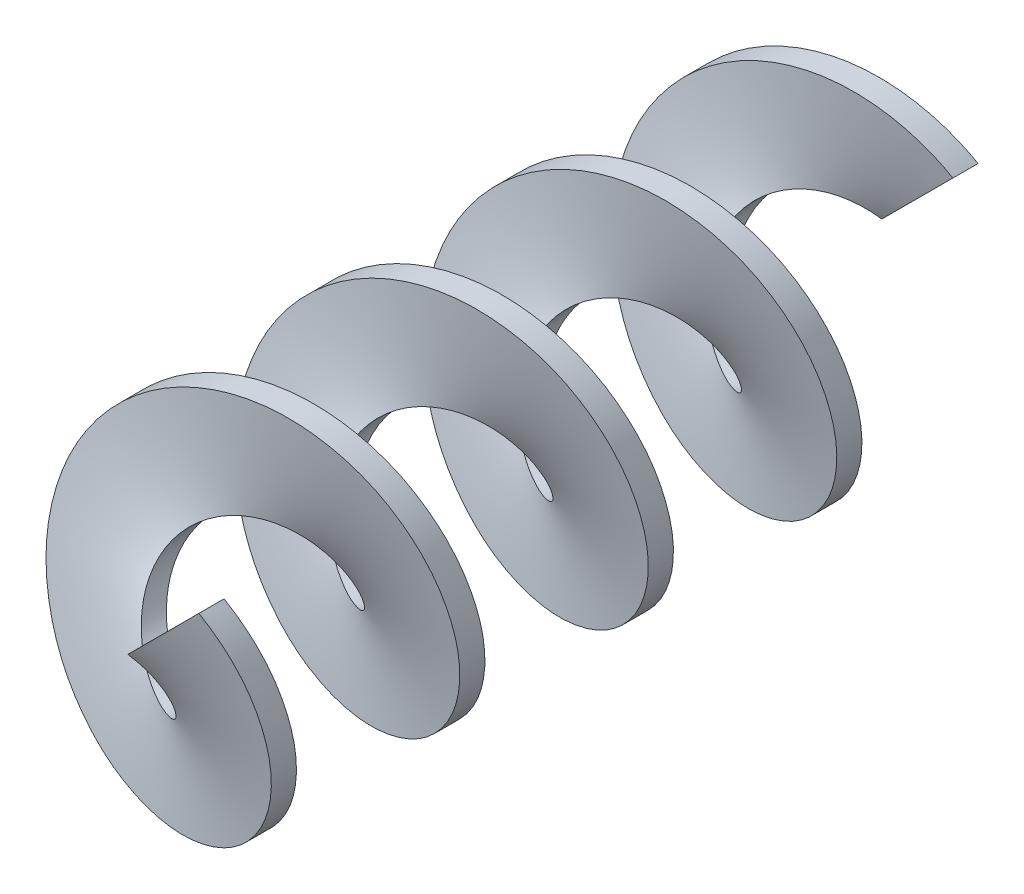
SolidWorks part; units mm, degrees
ref_plane "Front Plane" through (0, 0, 0) normal (0, 0, 1) x (1, 0, 0)
ref_plane "Top Plane" through (0, 0, 0) normal (0, 1, 0) x (1, 0, 0)
ref_plane "Right Plane" through (0, 0, 0) normal (1, 0, 0) x (0, 0, -1)
ref_plane "Plane1" through (0, 0, 15) normal (0, 0, 1) x (1, 0, 0)
sketch "Sketch2" plane through (0, 0, 15) normal (0, 0, 1) x (1, 0, 0)
  circle A0 centre (0, 0) radius 3
  dimension "D1" = 6
curve "Helix/Spiral1" pitch 3.75 height 15 turns 4
sketch "Sketch16" plane through (0, 0, 0) normal (0, 1, 0) x (1, 0, 0)
  line L1 (3.1213, -14.75) -> (1.1213, -14.75)
  line L2 (3.1213, -14.75) -> (3.1213, -15.25)
  line L3 (3.1213, -15.25) -> (1.1213, -15.25)
  line L4 (1.1213, -14.75) -> (1.1213, -15.25)
  line L5 (3.1213, -14.75) -> (1.1213, -15.25) construction
  line L6 (3.1213, -15.25) -> (1.1213, -14.75) construction
  spline S0 degree 3 poles (2.1213, -15) (2.3973, -14.9224) (2.8446, -14.7654) (3.0779, -14.5313) (2.8439, -14.2969) (2.1765, -14.0625) (1.1779, -13.8281) (0, -13.5938) (-1.1779, -13.3594) (-2.1765, -13.125) (-2.8438, -12.8906) (-3.0781, -12.6563) (-2.8438, -12.4219) (-2.1765, -12.1875) (-0.8451, -11.875) (0.8451, -11.5625) (2.1765, -11.25) (2.8438, -11.0156) (3.0781, -10.7813) (2.8438, -10.5469) (2.1765, -10.3125) (0.8451, -10) (-0.8451, -9.6875) (-2.1765, -9.375) (-2.8438, -9.1406) (-3.0781, -8.9062) (-2.8438, -8.6719) (-2.1765, -8.4375) (-0.8451, -8.125) (0.8451, -7.8125) (2.1765, -7.5) (2.8438, -7.2656) (3.0781, -7.0312) (2.8438, -6.7969) (2.1765, -6.5625) (0.8451, -6.25) (-0.8451, -5.9375) (-2.1765, -5.625) (-2.8438, -5.3906) (-3.0781, -5.1562) (-2.8438, -4.9219) (-2.1765, -4.6875) (-0.8451, -4.375) (0.8451, -4.0625) (2.1765, -3.75) (2.8438, -3.5156) (3.0781, -3.2812) (2.8438, -3.0469) (2.1765, -2.8125) (0.8451, -2.5) (-0.8451, -2.1875) (-2.1765, -1.875) (-2.8438, -1.6406) (-3.0781, -1.4062) (-2.8438, -1.1719) (-2.1765, -0.9375) (-1.178, -0.7031) (0.0002, -0.4687) (1.1772, -0.2346) (1.8454, -0.0776) (2.1213, 0) knots 0 0 0 0 0.015625 0.03125 0.046875 0.0625 0.078125 0.09375 0.109375 0.125 0.140625 0.15625 0.171875 0.1875 0.203125 0.234375 0.25 0.265625 0.28125 0.296875 0.3125 0.328125 0.359375 0.375 0.390625 0.40625 0.421875 0.4375 0.453125 0.484375 0.5 0.515625 0.53125 0.546875 0.5625 0.578125 0.609375 0.625 0.640625 0.65625 0.671875 0.6875 0.703125 0.734375 0.75 0.765625 0.78125 0.796875 0.8125 0.828125 0.859375 0.875 0.890625 0.90625 0.921875 0.9375 0.953125 0.96875 0.984375 1 1 1 1 construction
  point P0 (2.1213, -15)
  dimension "D1" = 2
  dimension "D2" = 0.5
sweep "Sweep1" add profiles "Sketch16" path "Helix/Spiral1"
